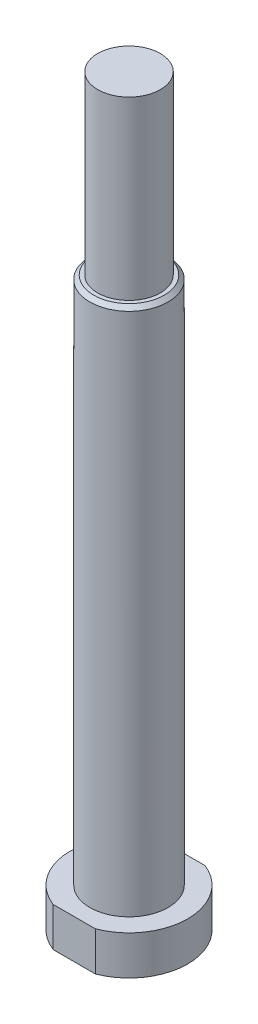
from build123d import *

# Parameters (mm, degrees)
CHAMFER_1_SIZE      = 1
SKETCH_2_W          = 36.885897288
SKETCH_2_H          = 4.926272709
SKETCH_2_W_2        = 40.411275082
SKETCH_2_H_2        = 4.776597597
CUT_EXTRUDE_1_DEPTH = 30


with BuildPart() as part:
    # 草图1 → 旋转1 (revolve)
    with BuildSketch(Plane.XY, mode=Mode.PRIVATE) as revolve_1_sk:
        Polygon((0, 95), (0, -95), (15, -95), (15, -85), (10, -85), (10, 50), (8, 50), (8, 95), align=None)
    revolve(revolve_1_sk.sketch.rotate(Axis((0, 95, 0), (0, -1, 0)), 180), axis=Axis((0, 95, 0), (0, -1, 0)))

    # 倒角1
    chamfer_1_edges = [part.edges().sort_by_distance(p)[0] for p in [
        (10, 50, 0),
    ]]
    chamfer(chamfer_1_edges, length=CHAMFER_1_SIZE)

    # 草图2 → 切除-拉伸1 (cut)
    with BuildSketch(Plane(origin=(0, -85, 0), x_dir=(1, 0, 0), z_dir=(0, 1, 0))):
        with Locations((-1.52363424, -16.463136355)):
            Rectangle(SKETCH_2_W, SKETCH_2_H)
        with Locations((0.239054657, 16.388298799)):
            Rectangle(SKETCH_2_W_2, SKETCH_2_H_2)
    extrude(amount=-CUT_EXTRUDE_1_DEPTH, mode=Mode.SUBTRACT)


solid = part.part
